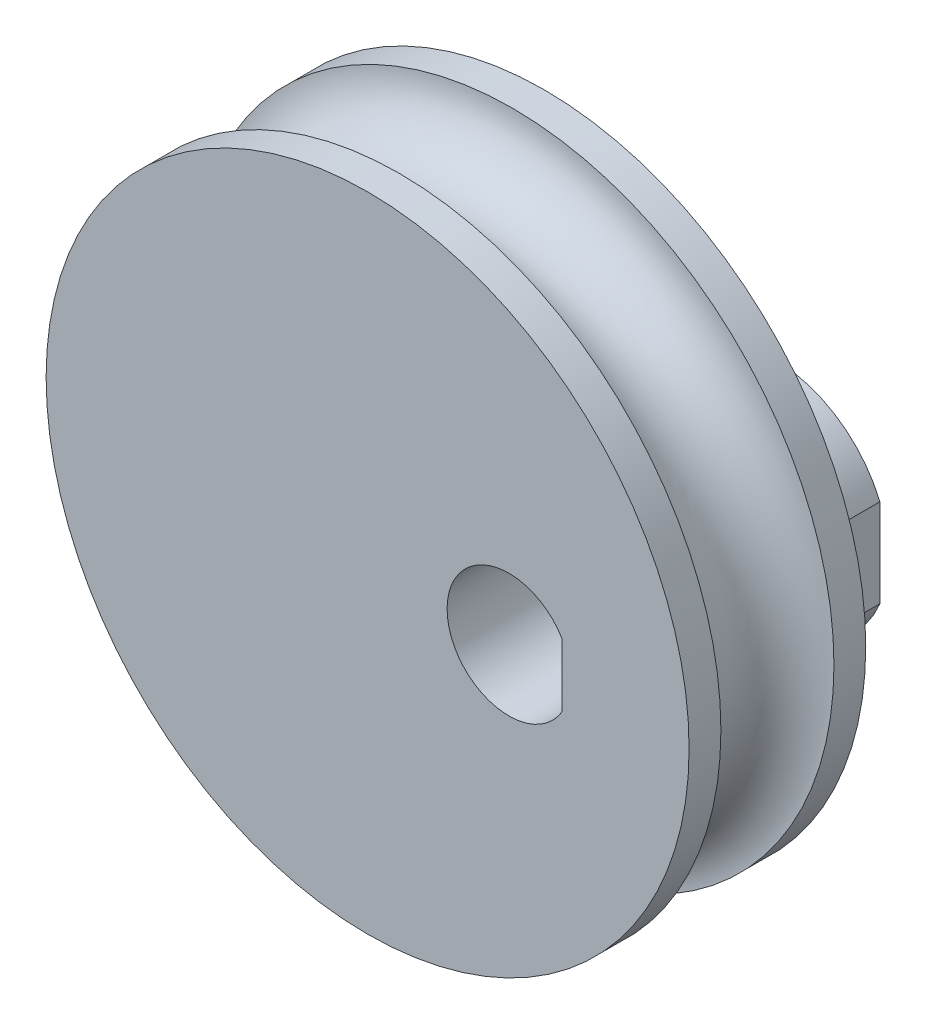
SolidWorks part; units mm, degrees
ref_plane "前视基准面" through (0, 0, 0) normal (0, 0, 1) x (1, 0, 0)
ref_plane "上视基准面" through (0, 0, 0) normal (0, 1, 0) x (1, 0, 0)
ref_plane "右视基准面" through (0, 0, 0) normal (1, 0, 0) x (0, 0, -1)
sketch "草图1" plane through (0, 0, 0) normal (0, 0, 1) x (1, 0, 0)
  line L0 (11, 1.8028) -> (11, -1.8028)
  line L1 (0, 0) -> (8, 0) construction
  circle A1 centre (8, 0) radius 3.5
  circle A2 centre (0, 0) radius 15
  dimension "D1" = 30
  dimension "D2" = 7
  dimension "D3" = 3
  dimension "D4" = 8
extrude "凸台-拉伸1" add sketch "草图1" along normal mid plane 10
sketch "草图4" plane through (0, 0, 0) normal (0, 1, 0) x (1, 0, 0)
  line L0 (15, 5) -> (15, -5)
  line L1 (15, -5) -> (18.2, -5)
  line L3 (18.2, 5) -> (15, 5)
  line L4 (0, 0) -> (18.2, 0) construction
  line L5 (0, 0) -> (0, 6.7467) construction
  line L6 (18.2, -3.2) -> (18.2, -5)
  line L7 (18.2, 3.2) -> (18.2, 5)
  arc A0 (18.2, 3.2) -> (18.2, -3.2) centre (18.2, 0) ccw
  dimension "D1" = 3.2
revolve "旋转1" add sketch "草图4" angle 360 about L5
sketch "草图5" plane through (0, 0, -5) normal (0, 0, 1) x (1, 0, 0)
  line L0 (14, -2.5) -> (14, 2.5)
  line L1 (11, -1.8028) -> (11, 1.8028)
  line L2 (11, -1.8028) -> (11, 1.8028)
  arc A1 (14, 2.5) -> (14, -2.5) centre (8, 0) ccw
  arc A2 (11, 1.8028) -> (11, -1.8028) centre (8, 0) ccw
  arc A3 (11, 1.8028) -> (11, -1.8028) centre (8, 0) ccw
  dimension "D1" = 0
  dimension "D2" = 3
extrude "凸台-拉伸2" add sketch "草图5" against normal blind 5
sketch "草图6" plane through (14, 0, 0) normal (1, 0, 0) x (0, 0, -1)
  line L0 (10, 0) -> (7.5, 0) construction
  line L1 (10, -2.5) -> (10, 2.5) construction
  line L2 (5, 0) -> (7.5, 0) construction
  line L3 (5, -18.2) -> (5, 18.2) construction
hole_wizard "M3x0.5 螺纹孔1" positions "3D草图1" profile "草图7" tap size "M3x0.5" standard "BSI"
sketch3d "3D草图1"
  point P0 (14, 0, -7.5)
sketch "草图7" plane through (14, 0, -7.5) normal (0, 1, 0) x (0, 0, -1)
  line L0 (0, 0) -> (0, 8.2511)
  line L1 (0, 8.2511) -> (1.25, 7.5)
  line L2 (1.25, 7.5) -> (1.25, 0)
  line L5 (1.25, 0) -> (0, 0)
  line L10 (0, 8.2511) -> (-1.25, 7.5) construction
  line L11 (0, -6.35) -> (0, 107.95) construction
  dimension "螺纹孔钻头直径" = 2.5
  dimension "螺纹孔钻头深度" = 7.5
  dimension "导头角度" = 118
cosmetic thread "孔螺蚊线1" parameters "D1"=3, "D2"=3
